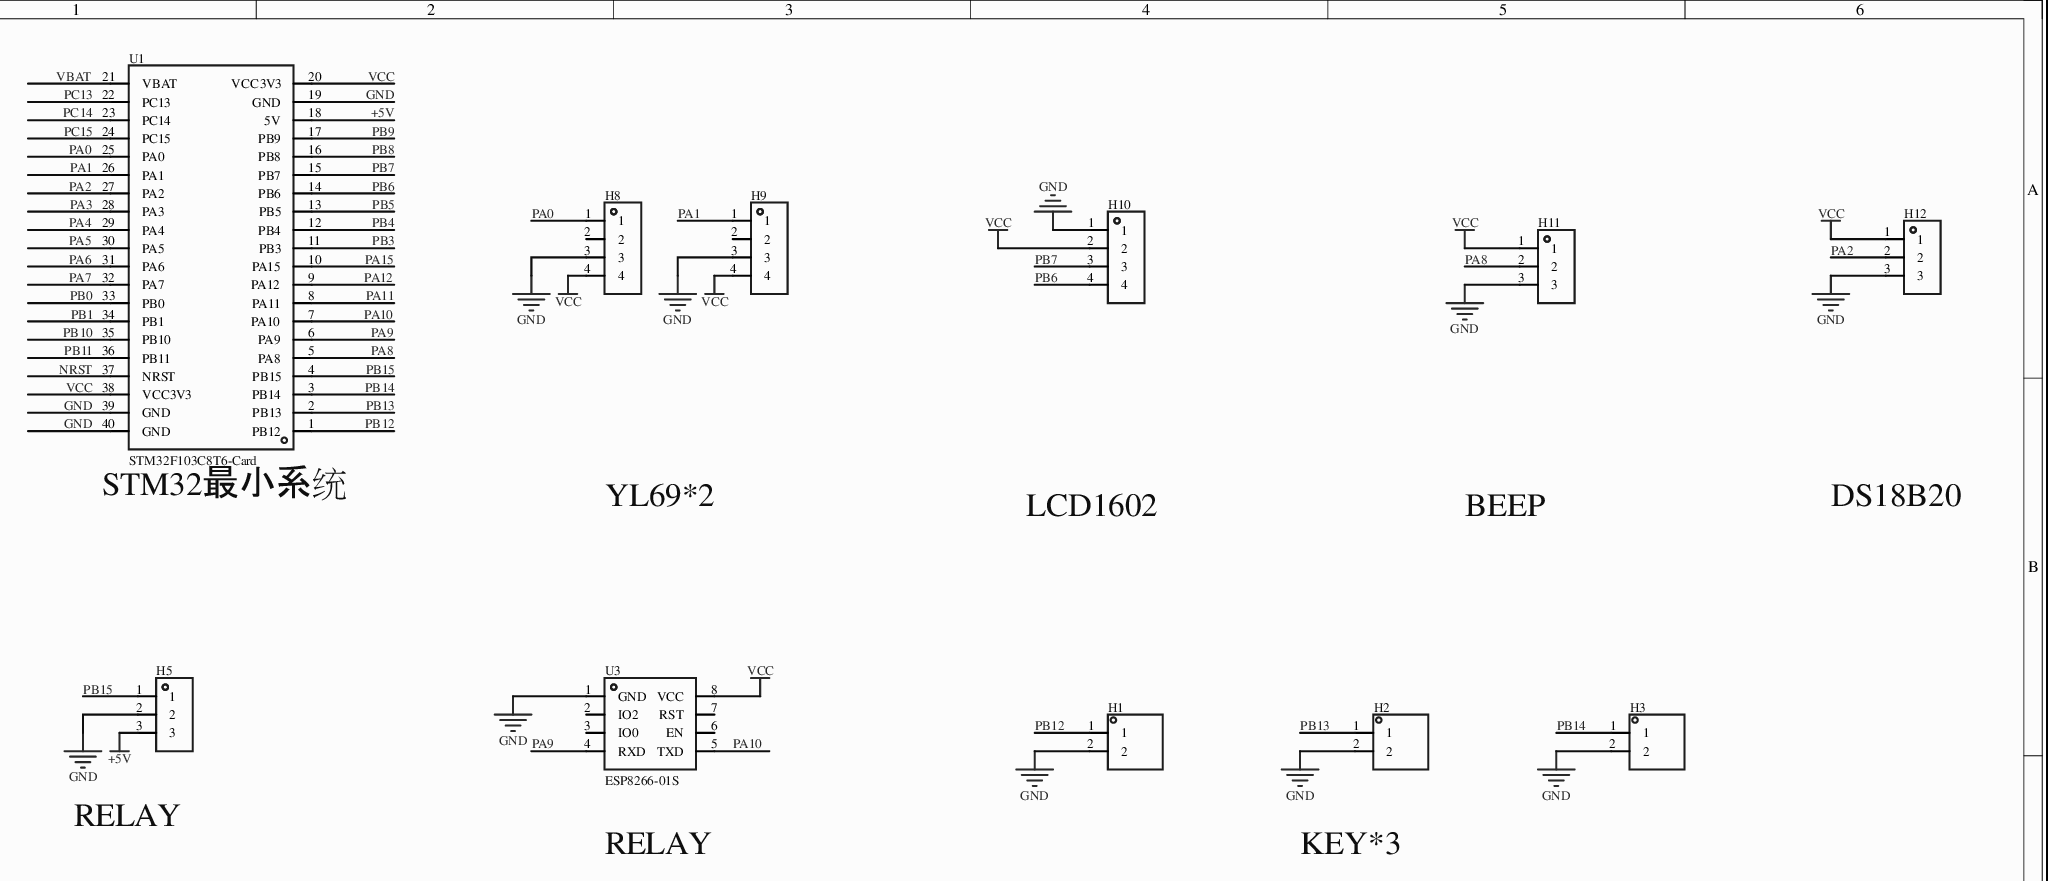
[diagram p0: MISC51268-3.schdoc]
# Altium project MISC51268-2.PrjPcb
1 sheet, 11 parts. Net scope: global (net labels, ports and power ports of the same name join across sheets).
Board file: MISC51268.pcbdoc

## Sheet MISC51268-3.schdoc
size 297 x 209 mm; Version: V1.0; @Project Name: MISC51268; @Page Count: 1; @Update Date: 2026-03-24; @Create Date: 2026-03-24; @Schematic Name: MISC51268; @Page No: 1; @Create Time: 18:58:15; @Update Time: 22:44:58; @Board Name: MISC51268

### Parts
H1  (no value)  [HDR-TH_2P-P2.54-V-M-1]
H2  (no value)  [HDR-TH_2P-P2.54-V-M-1]
H3  (no value)  [HDR-TH_2P-P2.54-V-M-1]
H5  (no value)  [HDR-TH_3P-P2.54-V-F]
H8  (no value)  [HDR-TH_4P-P2.54-V-F]
H9  (no value)  [HDR-TH_4P-P2.54-V-F]
H10  (no value)  [HDR-TH_4P-P2.54-V-F]
H11  (no value)  [HDR-TH_3P-P2.54-V-F]
H12  (no value)  [HDR-TH_3P-P2.54-V-F]
U1  STM32F103C8T6-Card  [CONN-TH_L53.3-W22.9_STM32F103C8T6-CARD]
U3  ESP8266-01S  [WIFIM-TH_ESP8266-01S]

### Nets
+5V: H5.3 U1.18(5V)
GND: H1.2 H2.2 H3.2 H5.2 H8.3 H9.3 H10.1 H11.3 H12.3 U1.19(GND) U1.39(GND) U1.40(GND) U3.1(GND)
VCC: H8.4 H9.4 H10.2 H11.1 H12.1 U1.20(VCC3V3) U1.38(VCC3V3) U3.8(VCC)
NRST: U1.37(NRST)
PA0: H8.1 U1.25(PA0)
PA1: H9.1 U1.26(PA1)
PA2: H12.2 U1.27(PA2)
PA3: U1.28(PA3)
PA4: U1.29(PA4)
PA5: U1.30(PA5)
PA6: U1.31(PA6)
PA7: U1.32(PA7)
PA8: H11.2 U1.5(PA8)
PA9: U1.6(PA9) U3.4(RXD)
PA10: U1.7(PA10) U3.5(TXD)
PA11: U1.8(PA11)
PA12: U1.9(PA12)
PA15: U1.10(PA15)
PB0: U1.33(PB0)
PB1: U1.34(PB1)
PB3: U1.11(PB3)
PB4: U1.12(PB4)
PB5: U1.13(PB5)
PB6: H10.4 U1.14(PB6)
PB7: H10.3 U1.15(PB7)
PB8: U1.16(PB8)
PB9: U1.17(PB9)
PB10: U1.35(PB10)
PB11: U1.36(PB11)
PB12: H1.1 U1.1(PB12)
PB13: H2.1 U1.2(PB13)
PB14: H3.1 U1.3(PB14)
PB15: H5.1 U1.4(PB15)
PC13: U1.22(PC13)
PC14: U1.23(PC14)
PC15: U1.24(PC15)
VBAT: U1.21(VBAT)

Not connected (* = marked no-connect by the designer): H8 2; H9 2; U3 2(IO2) 3(IO0) 6(EN) 7(RST)

### Notes on the sheet
- (near U1) STM32最小系统
- YL69*2
- LCD1602
- BEEP
- DS18B20
- (near H5) RELAY
- RELAY
- KEY*3

### Library data of the parts
H1-H3 = HDR-M_2.54_1x2P: Symbol: 210S-1*2P L=11.6MMGold-plated black; ConvertToPcb: yes; ModelId: 79b2e9f2d70a4d68a1b7098f27c6d4c50819f05c4eef4c71ace90d822a990e87; ModelName: HDR-M-2.54_1x2; ModelTransform: 200,100,0,0,0,0,0,0,-118.11; Device: HDR-M_2.54_1x2P; AddInBom: yes; SupplierPart: C124375; Supplier Footprint: 插件; FootprintName: HDR-TH_2P-P2.54-V-M-1
H5 H11 H12 = HDR-F_2.54_1x3P: Symbol: PM254V-11-03-H85; 3D Model: f3b3cc5aae9641bf9e56fc160cef875b; 3D Model Transform: 299.9994,100,0,0,0,0,0,0,-118.11; ConvertToPcb: yes; ModelName: HDR2.54-F-LI-1X3P; Device: HDR-F_2.54_1x3P; Supplier Part: C541850; Supplier Footprint: 插件; AddInBom: yes; FootprintName: HDR-TH_3P-P2.54-V-F
H8-H10 = HDR-F_2.54_1x4P: Symbol: 2.54-1*4P母; 3D Model: d187812051054f85879fcaa51a310d8e0819f05c4eef4c71ace90d822a990e87; 3D Model Transform: 419.6842,98.464,0,0,0,0,0,0,-118.11; ConvertToPcb: yes; Device: HDR-F_2.54_1x4P; Supplier Part: C2718488; Supplier Footprint: 插件; AddInBom: yes; FootprintName: HDR-TH_4P-P2.54-V-F; ModelName: HDR-TH_4P-P2.54-V-F
U1 = STM32F103C8T6-Card: AddInBom: yes; Symbol: STM32F103C8T6-CARD; Device: STM32F103C8T6-Card; LCSC Part Name: STM32F103C8T6-Card; SupplierPart: C9900077949; ManufacturerPart: STM32F103C8T6-Card; Supplier Footprint: 插件; Supplier: LCSC; ConvertToPcb: yes; FootprintName: CONN-TH_L53.3-W22.9_STM32F103C8T6-CARD
U3 = ESP8266-01S: AddInBom: yes; ModelId: 7671a3a19d0d4245ae5d5806b59f4d510819f05c4eef4c71ace90d822a990e87; ModelTransform: 566.928,972.439,0,0,0,0,0,378.464,-118.11; Symbol: ESP8266-01S; Device: ESP8266-01S; LCSC Part Name: ESP8266-01S; SupplierPart: C9900150497; ManufacturerPart: ESP8266-01S; Supplier Footprint: TH-8P; JLCPCB Part Class: Extended Part; Supplier: LCSC; ConvertToPcb: yes; FootprintName: WIFIM-TH_ESP8266-01S; ModelName: WIFIM-TH_ESP8266-01S